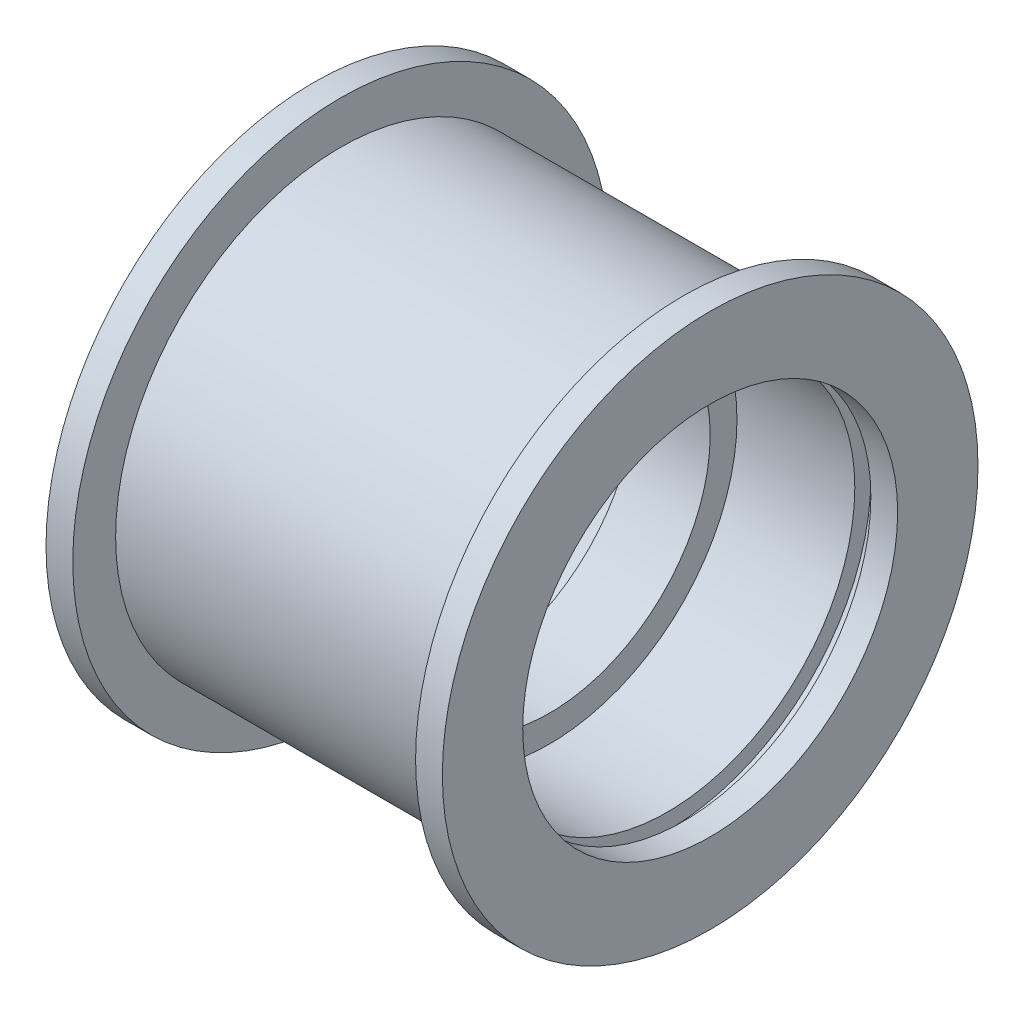
SolidWorks part; units mm, degrees
ref_plane "前视" through (0, 0, 0) normal (0, 0, 1) x (1, 0, 0)
ref_plane "上视" through (0, 0, 0) normal (0, 1, 0) x (1, 0, 0)
ref_plane "右视" through (0, 0, 0) normal (1, 0, 0) x (0, 0, -1)
sketch "草图1" plane through (0, 0, 0) normal (1, 0, 0) x (0, 0, -1)
  line L0 (0, 21) -> (0, 21.381) construction
  circle A1 centre (0, 0) radius 21
  circle A2 centre (0, 0) radius 21.381 construction
  dimension "D2" = 42
  dimension "D3" = 0.381
extrude "拉伸1" add sketch "草图1" along normal mid plane 32
sketch "草图2" plane through (16, 0, 0) normal (1, 0, 0) x (0, 0, -1)
  line L0 (0, 0) -> (0, 61.5267) construction
  line L1 (-3.285, 20.7415) -> (-1.8201, 17.6)
  line L2 (-1.8201, 17.6) -> (1.8201, 17.6)
  line L3 (1.8201, 17.6) -> (3.285, 20.7415)
  circle A0 centre (0, 0) radius 21 construction
  arc A1 (3.285, 20.7415) -> (-3.285, 20.7415) centre (0, 0) ccw
  dimension "D2" = 3.4
  dimension "D3" = 25
  dimension "D1" = 6.57
extrude "拉伸2" [suppressed] cut sketch "草图2" against normal up to surface (32 mm away)
fillet "圆角1" [suppressed] radius 0.6
fillet "圆角2" [suppressed] radius 0.8
pattern_circular "阵列(圆周)1" [suppressed] count 16 over 360
sketch "草图6" plane through (16, 0, 0) normal (1, 0, 0) x (0, 0, -1)
  circle A0 centre (0, 0) radius 25
  dimension "D1" = 50
extrude "凸台-拉伸2" add sketch "草图6" along normal blind 1.5
sketch "草图7" plane through (17.5, 0, 0) normal (1, 0, 0) x (0, 0, -1)
  circle A0 centre (0, 0) radius 25
  dimension "D1" = 50
extrude "凸台-拉伸3" add sketch "草图7" along normal blind 1
mirror "镜向2" about plane through (0, 0, 0) normal (1, 0, 0) of "凸台-拉伸3", "凸台-拉伸2"
sketch "草图8" plane through (-18.5, 0, 0) normal (-1, 0, 0) x (0, 0, 1)
  circle A0 centre (0, 0) radius 15
  dimension "D1" = 30
extrude "切除-拉伸1" cut sketch "草图8" against normal through all
sketch "草图9" plane through (-18.5, 0, 0) normal (-1, 0, 0) x (0, 0, 1)
  circle A0 centre (0, 0) radius 17.5
  dimension "D1" = 35
extrude "切除-拉伸2" cut sketch "草图9" against normal blind 15
sketch "草图10" plane through (0, 0, 0) normal (0, 1, 0) x (1, 0, 0)
  line L0 (-3.5, 17.5) -> (-18.5, 17.5) construction
  line L1 (-16, 17.5) -> (-14.5, 17.5)
  line L2 (-16, 17.5) -> (-16, 19)
  line L3 (-16, 19) -> (-14.5, 19)
  line L4 (-14.5, 17.5) -> (-14.5, 19)
  line L6 (0, 0) -> (-33.3455, 0) construction
  line L7 (-18.5, 25) -> (-18.5, -25) construction
  dimension "D1" = 1.5
  dimension "D2" = 4
  dimension "D3" = 19
revolve "切除-旋转1" cut sketch "草图10" angle 360 about L6
mirror "镜向3" about plane through (0, 0, 0) normal (1, 0, 0) of "切除-拉伸2", "切除-旋转1"
